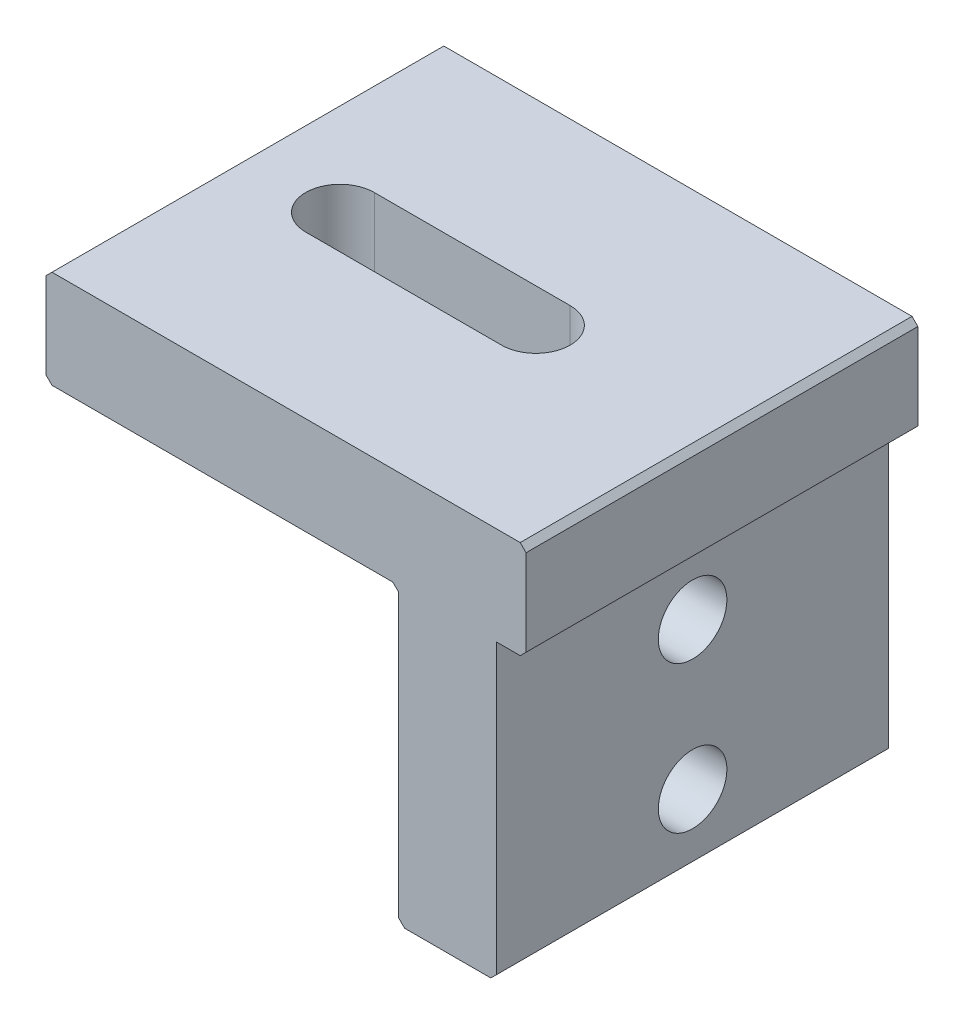
SolidWorks part; units mm, degrees
ref_plane "Front Plane" through (0, 0, 0) normal (0, 0, 1) x (1, 0, 0)
ref_plane "Top Plane" through (0, 0, 0) normal (0, 1, 0) x (1, 0, 0)
ref_plane "Right Plane" through (0, 0, 0) normal (1, 0, 0) x (0, 0, -1)
sketch "Sketch1" plane through (0, 0, 0) normal (0, 0, 1) x (1, 0, 0)
  line L0 (-6.8, 0) -> (-24.2, 0)
  line L1 (-0.3, 0) -> (-1.5, 0)
  line L2 (0, 0.3) -> (0, 4.7)
  line L3 (-0.3, 5) -> (-24.2, 5)
  line L4 (-24.5, 0.3) -> (-24.5, 4.7)
  line L6 (-6.5, -0.3) -> (-6.5, -14.7)
  line L7 (-6.2, -15) -> (-1.8, -15)
  line L8 (-1.5, 0) -> (-1.5, -14.7)
  line L9 (-24.2, 5) -> (-24.5, 4.7)
  line L10 (-24.2, 0) -> (-24.5, 0.3)
  line L11 (0, 4.7) -> (-0.3, 5)
  line L12 (0, 0.3) -> (-0.3, 0)
  line L13 (-6.5, -14.7) -> (-6.2, -15)
  line L14 (-1.8, -15) -> (-1.5, -14.7)
  line L15 (-6.5, -0.3) -> (-6.8, 0)
  point P0 (0, 0)
  point P1 (-24.5, 5)
  point P2 (0, 5)
  point P3 (-24.5, 0)
  point P5 (-6.5, 0)
  point P6 (-1.5, -15)
  point P7 (-6.5, -15)
  dimension "D1" = 5
  dimension "D2" = 5
  dimension "D3" = 1.5
  dimension "D4" = 15
  dimension "D5" = 18
extrude "Boss-Extrude1" add sketch "Sketch1" along normal blind 20
sketch "Sketch2" plane through (-1.5, 0, 0) normal (1, 0, 0) x (0, 0, -1)
  line L0 (-10, -14.7) -> (-10, 10.4373) construction
  line L1 (-20, -14.7) -> (0, -14.7) construction
  line L2 (0, -7.35) -> (-27.6392, -7.35) construction
  line L3 (0, -14.7) -> (0, 0) construction
  line L7 (-20, -15) -> (0, -15) construction
  circle A0 centre (-10, -11.5) radius 1.75
  circle A1 centre (-10, -4) radius 1.75
  dimension "D1" = 7.5
  dimension "D2" = 3.5
  dimension "D3" = 3.5
extrude "Cut-Extrude2" cut sketch "Sketch2" against normal up to next
sketch "Sketch5" plane through (0, 0, 0) normal (0, -1, 0) x (1, 0, 0)
  line L0 (-24.5, 10) -> (2.4856, 10) construction
  line L1 (-24.5, 20) -> (-24.5, 0) construction
  line L2 (-19.5, 10) -> (-9.5, 10) construction
  line L3 (-19.5, 11.75) -> (-9.5, 11.75)
  line L4 (-19.5, 8.25) -> (-9.5, 8.25)
  arc A0 (-19.5, 11.75) -> (-19.5, 8.25) centre (-19.5, 10) ccw
  arc A1 (-9.5, 8.25) -> (-9.5, 11.75) centre (-9.5, 10) ccw
  point P6 (-14.5, 10)
  dimension "D1" = 1.75
  dimension "D2" = 10
  dimension "D3" = 5
extrude "Cut-Extrude3" cut sketch "Sketch5" against normal up to next
